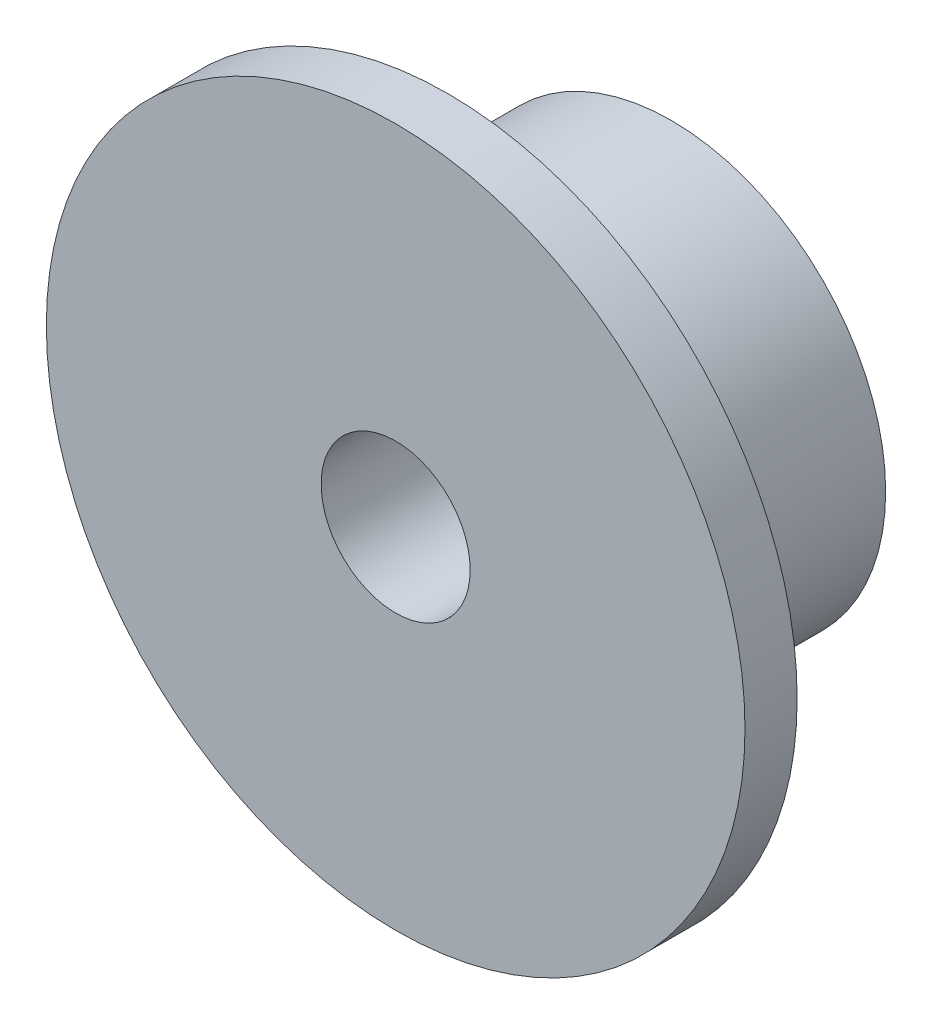
from build123d import *

# Parameters (mm, degrees)
SKETCH_1_R      = 11.5
SKETCH_1_R_2    = 4
EXTRUDE_1_DEPTH = 12
SKETCH_2_R      = 18.75
SKETCH_2_R_2    = 4
EXTRUDE_2_DEPTH = 2.8


with BuildPart() as part:
    # 草图1 → 凸台-拉伸1 (new body)
    with BuildSketch(Plane.XY):
        Circle(SKETCH_1_R)
        Circle(SKETCH_1_R_2, mode=Mode.SUBTRACT)
    extrude(amount=EXTRUDE_1_DEPTH)

    # 草图2 → 凸台-拉伸2 (add)
    with BuildSketch(Plane.XY.offset(12)):
        Circle(SKETCH_2_R)
        Circle(SKETCH_2_R_2, mode=Mode.SUBTRACT)
    extrude(amount=EXTRUDE_2_DEPTH)


solid = part.part
